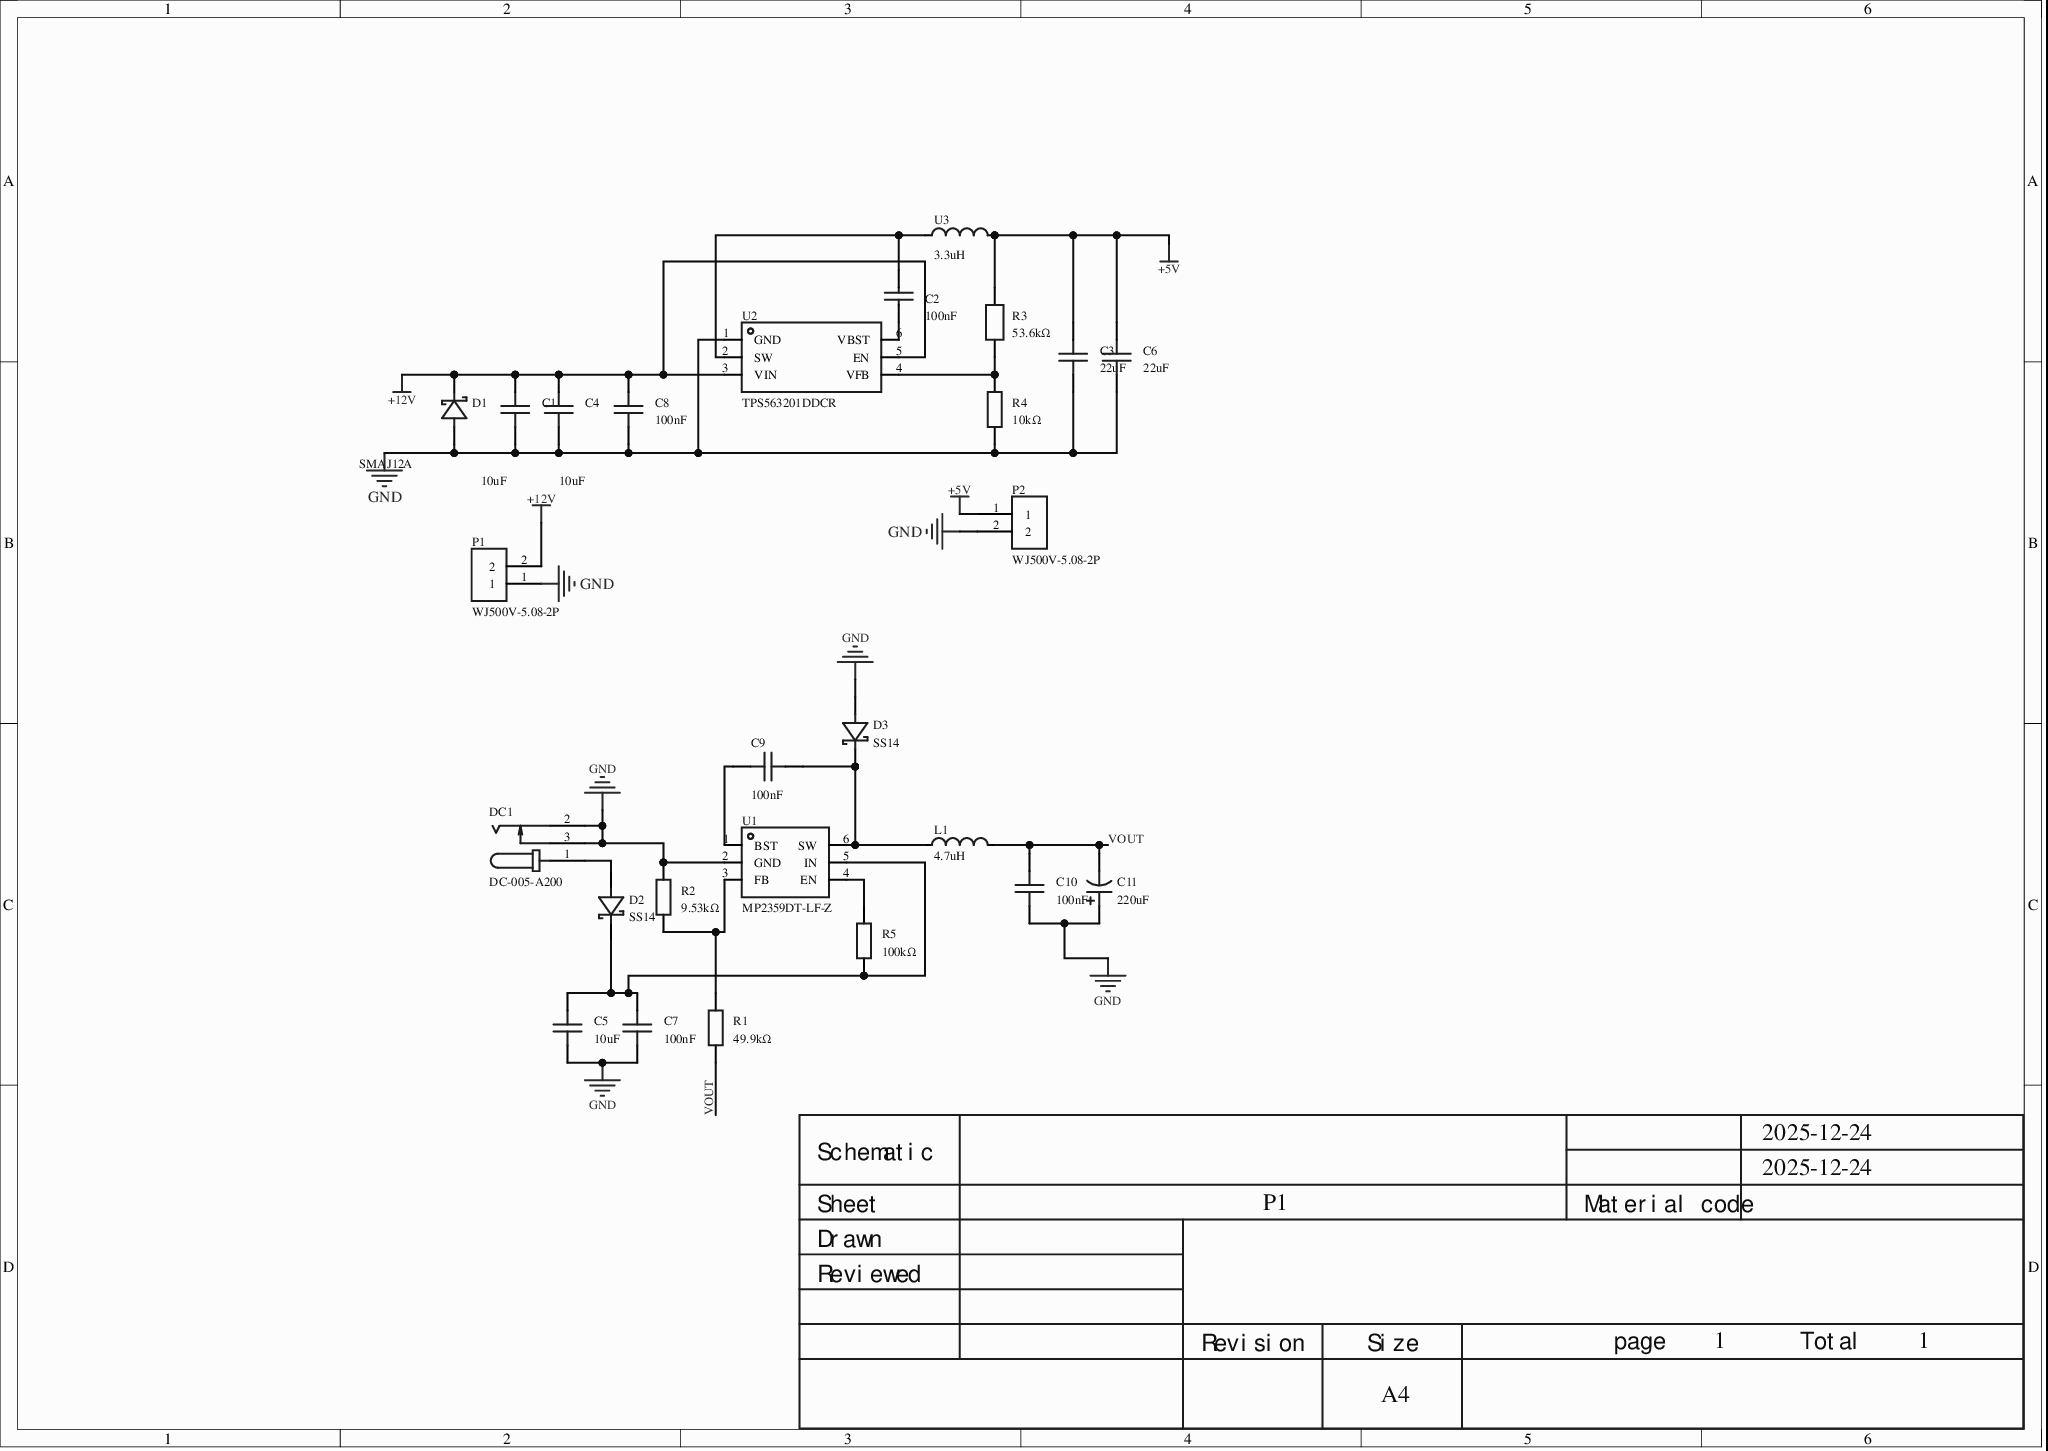
[diagram p0: MISC49894-3.schdoc]
# Altium project MISC49894-2.PrjPcb
1 sheet, 26 parts. Net scope: global (net labels, ports and power ports of the same name join across sheets).
Board file: MISC49894.pcbdoc

## Sheet MISC49894-3.schdoc
size 297 x 210 mm; Version: V1.0; @Project Name: MISC49894; @Page Count: 1; @Update Date: 2025-12-24; @Create Date: 2025-12-24; @Schematic Name: MISC49894; @Page No: 1; @Board Name: MISC49894; @Create Time: 11:08:26; @Update Time: 22:49:08

### Parts
C1  10uF  [C0805]
C2  100nF  [C0603]
C3  22uF  [C0603]
C4  10uF  [C0805]
C5  10uF  [C0603]
C6  22uF  [C0603]
C7  100nF  [C0603]
C8  100nF  [C0603]
C9  100nF  [C0603]
C10  100nF  [C0603]
C11  220uF  [CAP-SMD_BD10.0-L10.3-W10.3-LS11.7-FD]
D1  SMAJ12A  [DO-214AC_L4.3-W2.7-LS5.0-RD]
D2  SS14  [SMA_L4.3-W2.6-LS5.0-FD]
D3  SS14  [SMA_L4.3-W2.6-LS5.0-FD]
DC1  DC-005-A200  [DC-IN-TH_DC-005-A200]
L1  4.7uH  [L0603]
P1  WJ500V-5.08-2P  [CONN-TH_2P-P5.00_WJ500V-5.08-2P]
P2  WJ500V-5.08-2P  [CONN-TH_2P-P5.00_WJ500V-5.08-2P]
R1  49.9kΩ  [R0603]
R2  9.53kΩ  [R0603]
R3  53.6kΩ  [R0603]
R4  10kΩ  [R0603]
R5  100kΩ  [R0603]
U1  MP2359DT-LF-Z  [SOT-23-6_L2.9-W1.6-P0.95-LS2.8-BR]
U2  TPS563201DDCR  [SOT-23-6_L2.9-W1.6-P0.95-LS2.8-BR]
U3  3.3uH  [IND-SMD_L7.4-W6.6]

### Nets
+5V: C3.2 C6.2 P2.1 R3.2 U3.2
+12V: C1.2 C4.2 C8.2 D1.1(K) P1.2 U2.3(VIN) U2.5(EN)
GND: C1.1 C3.1 C4.1 C5.1 C6.1 C7.1 C8.1 C10.1 C11.1 D1.2(A) D3.1(A) DC1.2 DC1.3 P1.1 P2.2 R2.1 R4.1 U1.2(GND) U2.1(GND)
VOUT: C10.2 C11.2 L1.2 R1.2
NetC2_1: C2.1 U2.2(SW) U3.1
NetC2_2: C2.2 U2.6(VBST)
NetC5_2: C5.2 C7.2 D2.2(K) R5.2 U1.5(IN)
NetC9_1: C9.1 U1.1(BST)
NetC9_2: C9.2 D3.2(K) L1.1 U1.6(SW)
NetD2_1: D2.1(A) DC1.1
NetR1_1: R1.1 R2.2 U1.3(FB)
NetR3_1: R3.1 R4.2 U2.4(VFB)
NetR5_1: R5.1 U1.4(EN)

### Notes on the sheet
- 2025-12-24
- Schematic
- Sheet
- P1
- Material code
- Reviewed
- Drawn
- Revision
- Size
- A4
- page
- 1
- Total

### Library data of the parts
C1 C4 = CGA0805X5R106K350MT: Capacitance: 10uF; Tolerance: ±10%; Rated voltage: 35V; Dielectric (temp. coefficient): X5R;; Manufacturer: HRE(芯声); AddInBom: yes; ModelId: 1ba041120af144c991958decab20d241; ModelName: C0805_L2.0-W1.3-H1.3; ModelTransform: 78.74,51.181,0,0,0,0,0,0.0005,0; Symbol: CGA0805X5R106K350MT; Device: CGA0805X5R106K350MT; LCSC Part Name: 10uF ±10% 35V; SupplierPart: C6119888; ManufacturerPart: CGA0805X5R106K350MT; Supplier Footprint: 0805; JLCPCB Part Class: Extended library; Supplier: LCSC; ConvertToPcb: yes; FootprintName: C0805; Value: 10uF; Voltage Rated: 35V; Temperature Coefficient: X5R
C2 = CL10B104KA8NNNC: Capacitance: 100nF; Tolerance: ±10%; Rated voltage: 25V; Dielectric (temp. coefficient): X7R;; Manufacturer: SAMSUNG(三星); AddInBom: yes; ModelId: ac125912035d415993ca9572d50418b1; ModelName: C0603_L1.6-W0.8-H0.8; ModelTransform: 62.992,31.496,0,0,0,0,0,0,0; Symbol: CL10B104KA8NNNC; Device: CL10B104KA8NNNC; LCSC Part Name: 100nF ±10% 25V; SupplierPart: C1590; ManufacturerPart: CL10B104KA8NNNC; Supplier Footprint: 0603; JLCPCB Part Class: Extended library; Datasheet: example.com/upload/public/pdf/source/20160218/1457707763339.pdf; Supplier: LCSC; ConvertToPcb: yes; FootprintName: C0603; Value: 100nF; Voltage Rated: 25V; Temperature Coefficient: X7R
C3 C6 = HGC0603R5226M100NTHJ: Capacitance: 22uF; Tolerance: ±20%; Rated voltage: 10V; Dielectric (temp. coefficient): X5R;; Manufacturer: Chinocera(华瓷); AddInBom: yes; ModelId: ac125912035d415993ca9572d50418b1; ModelName: C0603_L1.6-W0.8-H0.8; ModelTransform: 62.992,31.496,0,0,0,0,0,0,0; Symbol: HGC0603R5226M100NTHJ; Device: HGC0603R5226M100NTHJ; LCSC Part Name: 22uF ±20% 10V; SupplierPart: C7432770; ManufacturerPart: HGC0603R5226M100NTHJ; Supplier Footprint: 0603; JLCPCB Part Class: Extended library; Datasheet: example.com/upload/public/pdf/source/20240320/FAC3FEC40A78BC5CCCE96C232A94D860.pdf; Supplier: LCSC; ConvertToPcb: yes; FootprintName: C0603; Value: 22uF; Voltage Rated: 10V; Temperature Coefficient: X5R
C5 = CGA0603X5R106K100JT: Capacitance: 10uF; Tolerance: ±10%; Rated voltage: 10V; Dielectric (temp. coefficient): X5R;; Manufacturer: HRE(芯声); AddInBom: yes; ModelId: ac125912035d415993ca9572d50418b1; ModelName: C0603_L1.6-W0.8-H0.8; ModelTransform: 62.992,31.496,0,0,0,0,0,0,0; Symbol: CGA0603X5R106K100JT; Device: CGA0603X5R106K100JT; LCSC Part Name: 10uF ±10% 10V; SupplierPart: C6119842; ManufacturerPart: CGA0603X5R106K100JT; Supplier Footprint: 0603; JLCPCB Part Class: Extended Part; Supplier: LCSC; ConvertToPcb: yes; FootprintName: C0603; Value: 10uF; Voltage Rated: 10V; Temperature Coefficient: X5R
C7 C9 C10 = CGA0603X7R104K500JT: Capacitance: 100nF; Tolerance: ±10%; Rated voltage: 50V; Dielectric (temp. coefficient): X7R;; Manufacturer: HRE(芯声); 3D Model: ac125912035d415993ca9572d50418b1; 3D Model Transform: 62.992,31.496,0,0,0,0,0,0,0; AddInBom: yes; ModelName: C0603_L1.6-W0.8-H0.8; Symbol: CGA0603X7R104K500JT; Device: CGA0603X7R104K500JT; LCSC Part Name: 100nF ±10% 50V; Supplier Part: C6119867; Manufacturer Part: CGA0603X7R104K500JT; Supplier Footprint: 0603; JLCPCB Part Class: Extended library; Supplier: LCSC; Value: 100nF; Voltage Rated: 50V; Temperature Coefficient: X7R; ConvertToPcb: yes; FootprintName: C0603
C8 = CGA0603X7R104K500JT: Capacitance: 100nF; Tolerance: ±10%; Rated voltage: 50V; Dielectric (temp. coefficient): X7R;; Manufacturer: HRE(芯声); AddInBom: yes; ModelId: ac125912035d415993ca9572d50418b1; ModelName: C0603_L1.6-W0.8-H0.8; ModelTransform: 62.992,31.496,0,0,0,0,0,0,0; Symbol: CGA0603X7R104K500JT; Device: CGA0603X7R104K500JT; LCSC Part Name: 100nF ±10% 50V; SupplierPart: C6119867; ManufacturerPart: CGA0603X7R104K500JT; Supplier Footprint: 0603; JLCPCB Part Class: Extended library; Supplier: LCSC; ConvertToPcb: yes; FootprintName: C0603; Value: 100nF; Voltage Rated: 50V; Temperature Coefficient: X7R
C11 = JVJ50V220M10x10: Capacitance: 220uF; Tolerance: ±20%; Rated voltage: 50V; Ripple current: 220mA@120Hz;; Manufacturer: JIERR(捷而瑞); AddInBom: yes; ModelId: 50f22ba8977a4cb2b51f8d950fa665c30819f05c4eef4c71ace90d822a990e87; ModelTransform: 456.692,405.511,0,0,0,0,0,0,0; Lifetime: 2000hrs@105℃; Symbol: JVJ50V220M10X10; Device: JVJ50V220M10x10; LCSC Part Name: 220uF ±20% 50V; SupplierPart: C46550417; ManufacturerPart: JVJ50V220M10x10; Supplier Footprint: SMD,D10xL10.5mm; JLCPCB Part Class: Extended Part; Datasheet: example.com/datasheet/JVJ50V220M10x10/48680111.html; Supplier: LCSC; ConvertToPcb: yes; FootprintName: CAP-SMD_BD10.0-L10.3-W10.3-LS11.7-FD; ModelName: CAP-SMD_BD10.0-L10.3-W10.3-LS11.7-FD; Value: 220uF; Voltage Rating: 50V; Ripple Current: 220mA@120Hz; Diameter: 10mm; Height - Seated (Max): 10.5mm; Operating Temperature: -55℃~+105℃
D1 = SMAJ12A_C908766: Reverse standoff voltage (Vrwm): 12V; Max clamping voltage: 19.9V; Peak pulse current (Ipp): 20.1A; Peak pulse power (Ppp): 400W; Breakdown voltage: 13.3V;; Manufacturer: GOODWORK(固得沃克); AddInBom: yes; ModelId: 5ef00dfc638b4df8bbf52dfa55db0c84; ModelTransform: 198.4248,106.299,0,0,0,0,-0.005,0,0; Reverse Leakage Current (Ir): 5uA; Type: TVS; Symbol: SMAJ12A_C908766; Device: SMAJ12A_C908766; LCSC Part Name: 单向TVS 12V截止 20.1A峰值脉冲; SupplierPart: C908766; ManufacturerPart: SMAJ12A; Supplier Footprint: SMA(DO-214AC); JLCPCB Part Class: Extended library; Datasheet: example.com/upload/public/pdf/source/20240508/8B44FA02DF89A45C8C3EB0325515EF7C.pdf; Supplier: LCSC; ConvertToPcb: yes; FootprintName: DO-214AC_L4.3-W2.7-LS5.0-RD; ModelName: DO-214AC_L4.3-W2.7-LS5.0-RD; Reverse Stand-Off Voltage (Vrwm): 12V; Maximum Clamping Voltage: 19.9V; Peak Pulse Current (Ipp): 20.1A; Peak Pulse Power Dissipation (Ppp): 400W; Breakdown Voltage: 13.3V; Operating Temperature: -55℃~+150℃@(Tj)
D2 D3 = SS14_C7420316: Diode configuration: Single; Forward voltage (Vf): 550mV@1.0A; DC reverse voltage (Vr): 40V; Rectified current: 1A;; Manufacturer: R+O(宏嘉诚); AddInBom: yes; ModelId: 7e24bebe6cd74171ae8c9de6fc5b78aa0819f05c4eef4c71ace90d822a990e87; ModelTransform: 198.4248,103.5431,0,180,0,0,0,0,0; Reverse Leakage Current (Ir): 200uA@40V; Operating Junction Temperature Range: -55℃~+150℃; Non-Repetitive Peak Forward Surge Current: 30A; Symbol: SS14_C7420316; Device: SS14_C7420316; LCSC Part Name: 电压:40V 电流:1A; SupplierPart: C7420316; ManufacturerPart: SS14; Supplier Footprint: SMA(DO-214AC); JLCPCB Part Class: Extended Part; Datasheet: example.com/datasheet/SS14/8397138.html; Supplier: LCSC; ConvertToPcb: yes; FootprintName: SMA_L4.3-W2.6-LS5.0-FD; ModelName: SMA_L4.3-W2.6-LS5.0-FD; Diode Configuration: Single; Voltage - Forward(Vf@If): 550mV@1.0A; Voltage - DC Reverse(Vr): 40V; Current - Rectified: 1A
DC1 = DC-005-A200: Connector type: DC power jack; Mounting: right-angle; Contact inner diameter: 2mm; Contact outer diameter: 6.4mm; Rated current: 3A; Rated voltage: 30V; Operating temperature: -20℃~+70℃;; Manufacturer: XUNPU(讯普); AddInBom: yes; ModelId: 1321cdbe1dc84555a9684967491c86700819f05c4eef4c71ace90d822a990e87; ModelTransform: 553.149,368.14887,0,0,0,0,-137.795,85.63,-161.417; Symbol: DC-005-A200; Device: DC-005-A200; LCSC Part Name: DC电源插座 内径:2mm 外径:6.4mm; SupplierPart: C720557; ManufacturerPart: DC-005-A200; Supplier Footprint: 插件; JLCPCB Part Class: Extended Part; Datasheet: example.com/datasheet/DC-005-A200/763564.html; Supplier: LCSC; ConvertToPcb: yes; FootprintName: DC-IN-TH_DC-005-A200; ModelName: DC-IN-TH_DC-005-A200; Connector Type: DC power jack; Mounting Type: Right-angle; Inside Contact Diameter: 2mm; Outside Contact Diameter: 6.4mm; Current Rating: 3A; Voltage Rating (Max): 30V; Operating Temperature: -20℃~+70℃
L1 = LQM18PN4R7MFRL: Inductance: 4.7uH; Tolerance: ±20%; Rated current: 620mA; Saturation current (Isat): -; DC resistance (DCR): 440mΩ;; Manufacturer: muRata(村田); AddInBom: yes; ModelId: 2bc5ec593d464d6ba9807aec0b5673c20819f05c4eef4c71ace90d822a990e87; ModelName: L0603_L1.6-W0.8-H0.5_BEAD; ModelTransform: 62.992,31.496,0,180,0,0,0.094,0.629,0; Frequency - Self Resonant: 40MHz; Symbol: LQM18PN4R7MFRL; Device: LQM18PN4R7MFRL; LCSC Part Name: 4.7uH ±20%; SupplierPart: C114862; ManufacturerPart: LQM18PN4R7MFRL; Supplier Footprint: 0603; JLCPCB Part Class: Extended Part; Datasheet: example.com/datasheet/LQM18PN4R7MFRL/116106.html; Supplier: LCSC; ConvertToPcb: yes; FootprintName: L0603; Value: 4.7uH; Current Rating: 620mA; Current - Saturation (Isat): -; DC Resistance(DCR): 440mΩ; Q @ Frequency: -; Ratings: -
P1 P2 = WJ500V-5.08-2P: Structure: 1x2P; Pitch: 5.08mm; Colour: green; Mounting: through-hole; Rated current: 18A; Rated voltage: 250V; Rows: 1; Wire gauge - AWG: 14~30; Wire gauge - mm2: 2.5; Pins per row: 2; Contact material: -; Contact plating: -; Operating temperature range: -40℃~+105℃; Soldering temperature (max): -;; Manufacturer: KANGNEX(康奈克斯电气); Symbol: WJ500V-5.08-2P-14-00A; AddInBom: yes; ModelId: 0f4a503c8d3b4ae19ed61267f5e9a1d7; ModelTransform: 423.621,393.7,0,0,0,0,-11.811,19.685,-137.795; Wire Gauge - mm2: 2.5; Number of PINs Per Row: 2; Screw Specification: M2.5; Device: WJ500V-5.08-2P; LCSC Part Name: 1x2P 5.08mm 直插 排数:1 每排P数:2; SupplierPart: C8465; ManufacturerPart: WJ500V-5.08-2P; Supplier Footprint: 插件,P=5.08mm; JLCPCB Part Class: Extended library; Datasheet: example.com/upload/public/pdf/source/20191225/C8465_02D34CE5B5B4A53DF5891601D97FA9F4.pdf; Supplier: LCSC; ConvertToPcb: yes; FootprintName: CONN-TH_2P-P5.00_WJ500V-5.08-2P; ModelName: CONN-TH_2P-P5.00_WJ500V-5.08-2P; Color: Green; Mounting Style: Through-hole; Current Rating (Max): 18A; Voltage Rating (Max): 250V; Number of Pins: 2P; Number of Rows: 1; Wire Gauge - AWG: 14~30; Contact Material: -; Contact Plating: -; Operating Temperature Range: -40℃~+105℃; Soldering Temperature(Max): -
R1 = 0603WAF4992T5E: Resistor type: Thick-film resistor; Resistance: 49.9kΩ; Tolerance: ±1%; Power: 100mW; Working voltage: 75V; Temp. coefficient: ±100ppm/℃;; Manufacturer: UNI-ROYAL(厚声); AddInBom: yes; ModelId: fc143cca1e79419f9cd78b61e9279f080819f05c4eef4c71ace90d822a990e87; ModelTransform: 31.8897,63.7794,0,90,0,0,0,0,0; Symbol: 0603WAF4992T5E; Device: 0603WAF4992T5E; LCSC Part Name: 49.9kΩ ±1% 100mW 厚膜电阻; SupplierPart: C23184; ManufacturerPart: 0603WAF4992T5E; Supplier Footprint: 0603; JLCPCB Part Class: Basic Part; Datasheet: example.com/datasheet/0603WAF4992T5E/23911.html; Supplier: LCSC; ConvertToPcb: yes; FootprintName: R0603; ModelName: R0603; Type: Thick-film resistor; Value: 49.9kΩ; Power(Watts): 100mW; Voltage-Supply(Max): 75V; Temperature Coefficient: ±100ppm/℃; Operating Temperature: -55℃~+155℃
R2 = 0603WAF9531T5E: Resistor type: Thick-film resistor; Resistance: 9.53kΩ; Tolerance: ±1%; Power: 100mW; Max working voltage: 75V; Temp. coefficient: ±100ppm/℃;; Manufacturer: UNI-ROYAL(厚声); AddInBom: yes; ModelId: fc143cca1e79419f9cd78b61e9279f080819f05c4eef4c71ace90d822a990e87; ModelTransform: 31.8897,63.7794,0,90,0,0,0,0,0; Symbol: 0603WAF9531T5E; Device: 0603WAF9531T5E; LCSC Part Name: 9.53kΩ ±1% 100mW 厚膜电阻; SupplierPart: C23127; ManufacturerPart: 0603WAF9531T5E; Supplier Footprint: 0603; JLCPCB Part Class: Extended Part; Datasheet: example.com/upload/public/pdf/source/20200306/C422600_1E6D84923E4A46A82E41ADD87F860B5C.pdf; Supplier: LCSC; ConvertToPcb: yes; FootprintName: R0603; ModelName: R0603; Type: Thick-film resistor; Value: 9.53kΩ; Power(Watts): 100mW; Overload Voltage (Max): 75V; Temperature Coefficient: ±100ppm/℃; Operating Temperature Range: -55℃~+155℃
R3 = FRC0603F5362TS: Resistor type: Thick-film resistor; Resistance: 53.6kΩ; Tolerance: ±1%; Power: 100mW; Max working voltage: 75V; Temp. coefficient: ±100ppm/℃;; Manufacturer: FOJAN(富捷); AddInBom: yes; ModelId: fc143cca1e79419f9cd78b61e9279f08; ModelTransform: 31.8897,63.7794,0,90,0,0,0,0,0; Symbol: FRC0603F5362TS; Device: FRC0603F5362TS; LCSC Part Name: 53.6kΩ ±1% 100mW 厚膜电阻; SupplierPart: C2930115; ManufacturerPart: FRC0603F5362TS; Supplier Footprint: 0603; JLCPCB Part Class: Extended library; Datasheet: example.com/upload/public/pdf/source/20211221/925EC7D7225764EE0046F22065062C87.pdf; Supplier: LCSC; ConvertToPcb: yes; FootprintName: R0603; ModelName: R0603; Type: Thick-film resistor; Value: 53.6kΩ; Power(Watts): 100mW; Overload Voltage (Max): 75V; Temperature Coefficient: ±100ppm/℃; Operating Temperature Range: -55℃~+155℃
R4 = 0603WAF1002T5E: Resistor type: Thick-film resistor; Resistance: 10kΩ; Tolerance: ±1%; Power: 100mW; Max working voltage: 75V; Temp. coefficient: ±100ppm/℃;; Manufacturer: UNI-ROYAL(厚声); AddInBom: yes; ModelId: fc143cca1e79419f9cd78b61e9279f08; ModelTransform: 31.8897,63.7794,0,90,0,0,0,0,0; Symbol: 0603WAF1002T5E; Device: 0603WAF1002T5E; LCSC Part Name: 厚膜电阻 10kΩ ±1% 100mW; SupplierPart: C25804; ManufacturerPart: 0603WAF1002T5E; Supplier Footprint: 0603; JLCPCB Part Class: Basic library; Datasheet: example.com/upload/public/pdf/source/20200306/C422600_1E6D84923E4A46A82E41ADD87F860B5C.pdf; Supplier: LCSC; ConvertToPcb: yes; FootprintName: R0603; ModelName: R0603; Type: Thick-film resistor; Value: 10kΩ; Power(Watts): 100mW; Overload Voltage (Max): 75V; Temperature Coefficient: ±100ppm/℃; Operating Temperature Range: -55℃~+155℃
R5 = 0603WAF1003T5E: Resistor type: Thick-film resistor; Resistance: 100kΩ; Tolerance: ±1%; Power: 100mW; Working voltage: 75V; Temp. coefficient: ±100ppm/℃;; Manufacturer: UNI-ROYAL(厚声); AddInBom: yes; ModelId: fc143cca1e79419f9cd78b61e9279f080819f05c4eef4c71ace90d822a990e87; ModelTransform: 31.8897,63.7794,0,90,0,0,0,0,0; Symbol: 0603WAF1003T5E; Device: 0603WAF1003T5E; LCSC Part Name: 100kΩ ±1% 100mW 厚膜电阻; SupplierPart: C25803; ManufacturerPart: 0603WAF1003T5E; Supplier Footprint: 0603; JLCPCB Part Class: Basic Part; Datasheet: example.com/datasheet/0603WAF1003T5E/26546.html; Supplier: LCSC; ConvertToPcb: yes; FootprintName: R0603; ModelName: R0603; Type: Thick-film resistor; Value: 100kΩ; Power(Watts): 100mW; Voltage-Supply(Max): 75V; Temperature Coefficient: ±100ppm/℃; Operating Temperature: -55℃~+155℃
U1 = MP2359DT-LF-Z: Function type: Buck; Operating voltage: 4.5V~24V; Output voltage: 810mV~15V; Output current: 1.2A; Output type: Adjustable;; Manufacturer: MPS(芯源); AddInBom: yes; ModelId: 18da8f6c14a34920b3e136b5c401a1190819f05c4eef4c71ace90d822a990e87; ModelName: SOT-23-6_L2.9-W1.6-H1.5-LS2.8-P0.95; ModelTransform: 110.73671,114.173,0,180,0,0,0.001,-0.003,0; Frequency - Switching: 1.4MHz; Synchronous Rectifier: No; Number of Outputs: 1; Quiescent Current: 800uA; Switch tube (built-in/external): Built-in; Symbol: MP2359DT-LF-Z; Device: MP2359DT-LF-Z; LCSC Part Name: 采用TSOT23-6封装的1.2A、24V、1.4MHz降压转换器; SupplierPart: C6595509; ManufacturerPart: MP2359DT-LF-Z; Supplier Footprint: SOT-23-6; JLCPCB Part Class: Extended Part; Datasheet: example.com/datasheet/MP2359DT-LF-Z/7550404.html; Supplier: LCSC; ConvertToPcb: yes; FootprintName: SOT-23-6_L2.9-W1.6-P0.95-LS2.8-BR; Function: Buck; Voltage - Supply: 4.5V~24V; Output Voltage: 810mV~15V; Output Current: 1.2A; Operating Temperature: -40℃~+85℃@(TA); Topology: Buck; Output Type: Adjustable
U2 = TPS563201DDCR: Function type: Buck; Output type: Adjustable; Input voltage: 4.5V~17V; Output voltage: 768mV~7V; Output current: 3A;; Manufacturer: TI(德州仪器); AddInBom: yes; ModelId: 18da8f6c14a34920b3e136b5c401a119; ModelName: SOT-23-6_L2.9-W1.6-H1.5-LS2.8-P0.95; ModelTransform: 110.73671,114.173,0,180,0,0,0.001,-0.003,0; Switching Frequency: 580kHz; Number of Outputs: 1; Switch tube (built-in/external): Built-in; Symbol: TPS563201DDCR; Device: TPS563201DDCR; LCSC Part Name: 4.5V至17V输入,3A同步降压电压调节器; SupplierPart: C116592; ManufacturerPart: TPS563201DDCR; Supplier Footprint: SOT-23-THIN-6; JLCPCB Part Class: Extended library; Datasheet: example.com/upload/public/pdf/source/20230424/FEEFD13F14AFA838E4C009B2DDC1DFA0.pdf; Supplier: LCSC; ConvertToPcb: yes; FootprintName: SOT-23-6_L2.9-W1.6-P0.95-LS2.8-BR; Function: Buck; Output Type: Adjustable; Input Voltage: 4.5V~17V; Output Voltage: 768mV~7V; Output Current: 3A; Operating Temperature: -40℃~+125℃@(TJ); Synchronous Rectification: Yes; Topology: Buck
U3 = FDVE0630-H-3R3M=P3: Inductance: 3.3uH; Tolerance: ±20%; Rated current: 5.3A; Saturation current (Isat): -; DC resistance (DCR): 25.4mΩ;; Manufacturer: muRata(村田); AddInBom: yes; ModelId: 6ebe9088926641d898f5999c0d913d3a; ModelName: IND-SMD_L7.4-W6.6-H1.8; ModelTransform: 291.338,259.842,0,0,0,0,0,0,0; Symbol: FDVE0630-H-3R3M=P3; Device: FDVE0630-H-3R3M=P3; LCSC Part Name: 3.3uH ±20%; SupplierPart: C907934; ManufacturerPart: FDVE0630-H-3R3M=P3; Supplier Footprint: SMD,6.6x7.4mm; JLCPCB Part Class: Extended library; Datasheet: example.com/upload/public/pdf/source/20201022/C907934_A12BEBCEF0936F6BC4224EFDE20F99C5.pdf; Supplier: LCSC; ConvertToPcb: yes; FootprintName: IND-SMD_L7.4-W6.6; Value: 3.3uH; Rated Current: 5.3A; Saturation Current (Isat): -; DC Resistance (DCR): 25.4mΩ; Q @ Freq: -; Frequency - Self Resonant: -; Ratings: -